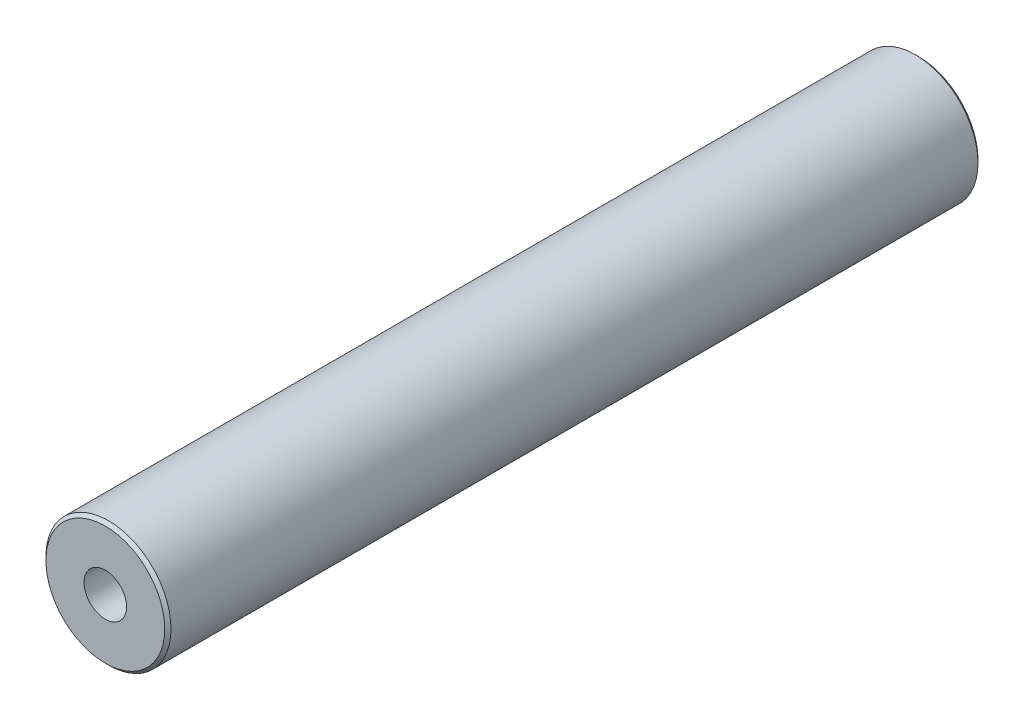
SolidWorks part; units mm, degrees
ref_plane "前视基准面" through (0, 0, 0) normal (0, 0, 1) x (1, 0, 0)
ref_plane "上视基准面" through (0, 0, 0) normal (0, 1, 0) x (1, 0, 0)
ref_plane "右视基准面" through (0, 0, 0) normal (1, 0, 0) x (0, 0, -1)
sketch "草图1" plane through (0, 0, 0) normal (0, 0, 1) x (1, 0, 0)
  circle A0 centre (0, 0) radius 10
  dimension "D1" = 20
extrude "凸台-拉伸1" add sketch "草图1" along normal blind 130
hole_wizard "M8 螺纹孔1" positions "草图3" profile "草图4" tap size "M8" standard "GB"
sketch "草图3" plane through (0, 0, 0) normal (0, 0, -1) x (-1, 0, 0)
  point P0 (0, 0)
sketch "草图4" plane through (0, 0, 0) normal (1, 0, 0) x (0, 1, 0)
  line L0 (0, 0) -> (0, 21.7929)
  line L1 (0, 21.7929) -> (3.4, 19.75)
  line L2 (3.4, 19.75) -> (3.4, 0)
  line L5 (3.4, 0) -> (0, 0)
  line L10 (0, 21.7929) -> (-3.4, 19.75) construction
  line L11 (0, -6.35) -> (0, 107.95) construction
  dimension "螺纹孔钻头直径" = 6.8
  dimension "螺纹孔钻头深度" = 19.75
  dimension "导头角度" = 118
cosmetic thread "孔螺蚊线1"
hole_wizard "M8 螺纹孔2" positions "草图6" profile "草图5" tap size "M8" standard "GB"
sketch "草图6" plane through (0, 0, 130) normal (0, 0, 1) x (1, 0, 0)
  point P0 (0, 0)
sketch "草图5" plane through (0, 0, 130) normal (1, 0, 0) x (0, -1, 0)
  line L0 (0, 0) -> (0, 21.7929)
  line L1 (0, 21.7929) -> (3.4, 19.75)
  line L2 (3.4, 19.75) -> (3.4, 0)
  line L5 (3.4, 0) -> (0, 0)
  line L10 (0, 21.7929) -> (-3.4, 19.75) construction
  line L11 (0, -6.35) -> (0, 107.95) construction
  dimension "螺纹孔钻头直径" = 6.8
  dimension "螺纹孔钻头深度" = 19.75
  dimension "导头角度" = 118
cosmetic thread "孔螺蚊线2"
chamfer "倒角1" distance 0.5 angle 45 2 edges at (10, 0, 0) (10, 0, 130)
